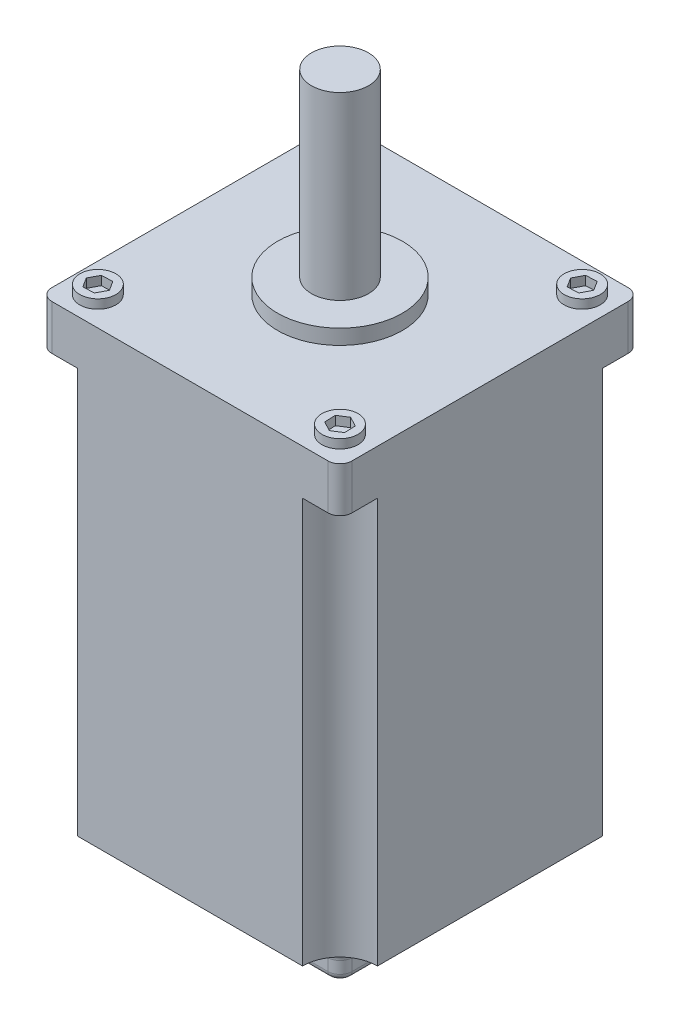
from build123d import *

# Parameters (mm, degrees)
SKETCH1_R           = 9.5
BOSS_EXTRUDE1_DEPTH = 60
SKETCH2_R           = 20.792572887
BOSS_EXTRUDE2_DEPTH = 5
SKETCH3_W           = 100
SKETCH3_H           = 100
BOSS_EXTRUDE3_DEPTH = 150
SKETCH4_R           = 12.5
CUT_EXTRUDE1_DEPTH  = 135
FILLET1_R           = 4
SKETCH5_W           = 78.706554356
SKETCH5_H           = 78.706554356
BOSS_EXTRUDE4_DEPTH = 10
FILLET2_R           = 4
FILLET3_R           = 2
SKETCH6_W           = 67.46675987
SKETCH6_H           = 9.193174248
CUT_EXTRUDE2_DEPTH  = 1.5
LPATTERN1_COUNT     = 6
LPATTERN1_PITCH     = 6.5
LPATTERN1_COL_COUNT = 6
LPATTERN1_COL_PITCH = 6.5
SKETCH7_R           = 6
BOSS_EXTRUDE5_DEPTH = 3
CIRPATTERN1_COUNT   = 4


with BuildPart() as part:
    # Sketch1 → Boss-Extrude1 (new body)
    with BuildSketch(Plane(origin=(0, 0, 0), x_dir=(1, 0, 0), z_dir=(0, 1, 0))):
        with Locations(Location((0, 0, 0), (0, 0, 270))):
            Circle(SKETCH1_R)
    extrude(amount=BOSS_EXTRUDE1_DEPTH)

    # Sketch2 → Boss-Extrude2 (add)
    with BuildSketch(Plane.XZ):
        with Locations(Location((0, 0, 0), (0, 0, 270))):
            Circle(SKETCH2_R)
    extrude(amount=BOSS_EXTRUDE2_DEPTH)

    # Sketch3 → Boss-Extrude3 (add)
    with BuildSketch(Plane.XZ.offset(5)):
        Rectangle(SKETCH3_W, SKETCH3_H)
    extrude(amount=BOSS_EXTRUDE3_DEPTH)

    # Sketch4 → Cut-Extrude1 (cut)
    with BuildSketch(Plane.XZ.offset(155)):
        with Locations((-50, 50)):
            Circle(SKETCH4_R)
        with Locations((50, 50)):
            Circle(SKETCH4_R)
        with Locations((-50, -50)):
            Circle(SKETCH4_R)
        with Locations((50, -50)):
            Circle(SKETCH4_R)
    extrude(amount=-CUT_EXTRUDE1_DEPTH, mode=Mode.SUBTRACT)

    # Fillet1
    fillet1_edges = [part.edges().sort_by_distance(p)[0] for p in [
        (50, -12.5, -50),
        (-50, -12.5, -50),
        (-50, -12.5, 50),
        (50, -12.5, 50),
    ]]
    fillet(fillet1_edges, radius=FILLET1_R)

    # Sketch5 → Boss-Extrude4 (add)
    with BuildSketch(Plane.XZ.offset(155)):
        Rectangle(SKETCH5_W, SKETCH5_H)
    extrude(amount=BOSS_EXTRUDE4_DEPTH)

    # Fillet2
    fillet2_edges = [part.edges().sort_by_distance(p)[0] for p in [
        (39.353277178, -155, 0),
        (39.353277178, -160, -39.353277178),
        (0, -155, 39.353277178),
        (39.353277178, -160, 39.353277178),
        (-39.353277178, -155, 0),
        (-39.353277178, -160, 39.353277178),
        (0, -155, -39.353277178),
        (-39.353277178, -160, -39.353277178),
    ]]
    fillet(fillet2_edges, radius=FILLET2_R)

    # Fillet3
    fillet3_edges = [part.edges().sort_by_distance(p)[0] for p in [
        (39.353277178, -165, 0),
        (0, -165, 39.353277178),
        (-39.353277178, -165, 0),
        (0, -165, -39.353277178),
        (38.181704302, -165, -38.181704302),
        (-38.181704302, -165, -38.181704302),
        (-38.181704302, -165, 38.181704302),
        (38.181704302, -165, 38.181704302),
    ]]
    fillet(fillet3_edges, radius=FILLET3_R)

    # Sketch6 → Cut-Extrude2 (cut, symmetric)
    with BuildSketch(Plane.XY):
        with Locations((0, -165)):
            Rectangle(SKETCH6_W, SKETCH6_H)
    cut_extrude2 = extrude(amount=CUT_EXTRUDE2_DEPTH, both=True, mode=Mode.SUBTRACT)

    # LPattern1: Cut-Extrude2 ×6
    with Locations(*[(0, 0, i * LPATTERN1_PITCH) for i in range(1, LPATTERN1_COUNT)]):
        add(cut_extrude2, mode=Mode.SUBTRACT)

    # LPattern1 col: Cut-Extrude2 ×6
    with Locations(*[(0, 0, -i * LPATTERN1_COL_PITCH) for i in range(1, LPATTERN1_COL_COUNT)]):
        add(cut_extrude2, mode=Mode.SUBTRACT)

    # Sketch7 → Boss-Extrude5 (add)
    with BuildSketch(Plane(origin=(0, -5, 0), x_dir=(1, 0, 0), z_dir=(0, 1, 0))):
        with Locations(Location((-40.343145751, 40.343145751, 0), (0, 0, 90))):
            Circle(SKETCH7_R)
        Polygon((-37.068403744, 38.622946456), (-37.216038458, 42.319055872), (-40.490780465, 44.039255167), (-43.617887757, 42.063345045), (-43.470253043, 38.367235629), (-40.195511036, 36.647036334), align=None, mode=Mode.SUBTRACT)
    boss_extrude5 = extrude(amount=BOSS_EXTRUDE5_DEPTH)

    # CirPattern1: Boss-Extrude5 ×4 about axis
    cirpattern1_axis = Axis((0, 0, 0), (0, 1, 0))
    for i in range(1, CIRPATTERN1_COUNT):
        add(boss_extrude5.rotate(cirpattern1_axis, i * 360 / CIRPATTERN1_COUNT))


solid = part.part
